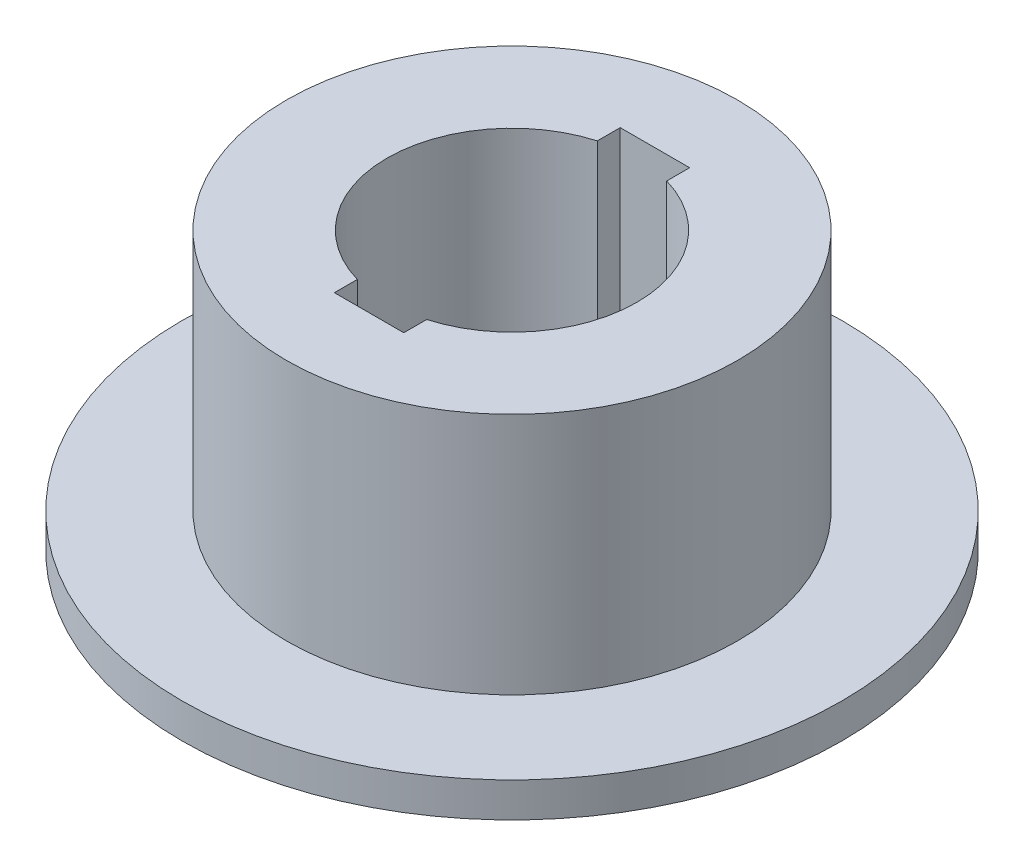
from build123d import *

# Parameters (mm, degrees)
SKETCH_1_R      = 32.500096928
EXTRUDE_1_DEPTH = 40
SKETCH_2_R      = 47.5
SKETCH_2_R_2    = 32.5
EXTRUDE_2_DEPTH = 5


with BuildPart() as part:
    # 草图1 → 凸台-拉伸1 (new body)
    with BuildSketch(Plane(origin=(0, 0, 0), x_dir=(1, 0, 0), z_dir=(0, 1, 0))):
        with Locations(Location((0, 0, 0), (0, 0, 270))):
            Circle(SKETCH_1_R)
        with BuildLine():
            Line((0, 20.591616466), (5, 20.591616466))
            Line((5, 20.591616466), (5, 17.291616466))
            ThreePointArc((5, 17.291616466), (18, 0), (5, -17.291616466))
            Line((5, -17.291616466), (5, -20.591616466))
            Line((5, -20.591616466), (0, -20.591616466))
            Line((0, -20.591616466), (-5, -20.591616466))
            Line((-5, -20.591616466), (-5, -17.291616466))
            ThreePointArc((-5, -17.291616466), (-18, 0), (-5, 17.291616466))
            Line((-5, 17.291616466), (-5, 20.591616466))
            Line((-5, 20.591616466), (0, 20.591616466))
        make_face(mode=Mode.SUBTRACT)
    extrude(amount=EXTRUDE_1_DEPTH)

    # 草图2 → 凸台-拉伸2 (add)
    with BuildSketch(Plane.XZ):
        with Locations(Location((0, 0, 0), (0, 0, 270))):
            Circle(SKETCH_2_R)
        Circle(SKETCH_2_R_2, mode=Mode.SUBTRACT)
    extrude(amount=-EXTRUDE_2_DEPTH)


solid = part.part
